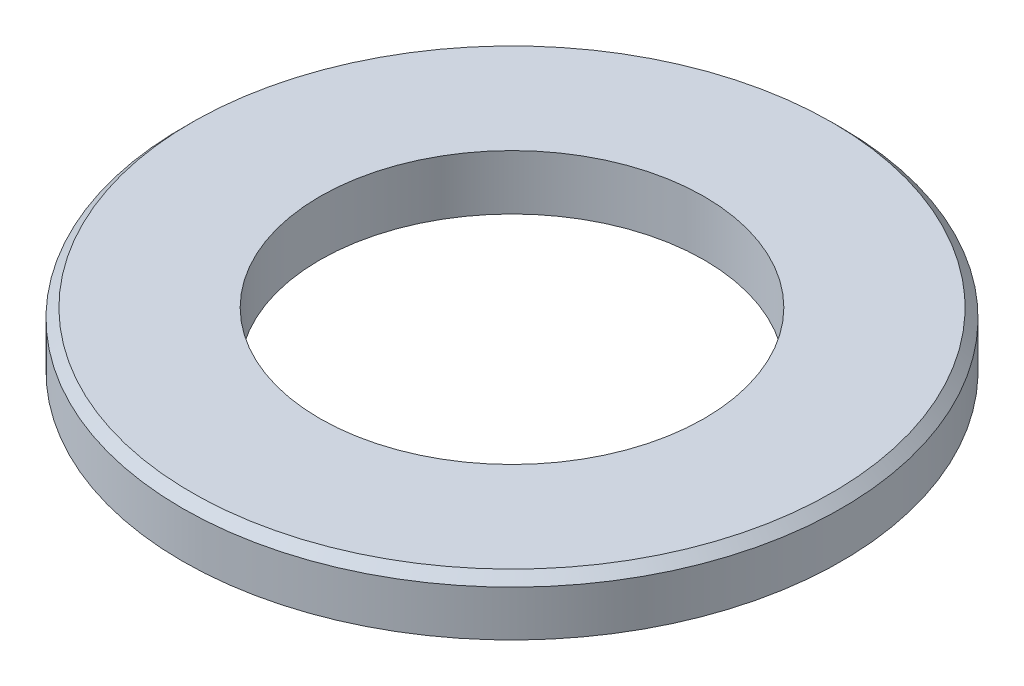
SolidWorks part; units mm, degrees
material "65Mn"
ref_plane "Plane1" through (0, 0, 0) normal (0, 0, 1) x (1, 0, 0)
ref_plane "Plane2" through (0, 0, 0) normal (0, 1, 0) x (1, 0, 0)
ref_plane "Plane3" through (0, 0, 0) normal (1, 0, 0) x (0, 0, -1)
sketch "Dimension sketch" plane through (0, 0, 0) normal (0, 0, 1) x (1, 0, 0)
  line L0 (0, 0) -> (9.1, 0)
  point P3 (4, 0)
  point P4 (56, 0)
  point P5 (31, 0)
  dimension "h" = 4
  dimension "d2" = 56
  dimension "d1" = 31
sketch "Sketch1" plane through (0, 0, 0) normal (0, 0, 1) x (1, 0, 0)
  line L0 (0, 0) -> (0, 52.7318) construction
  line L1 (-35, 14.6445) -> (-36, 13.6445)
  line L2 (-21, 8.6445) -> (-36, 8.6445)
  line L3 (-21, 8.6445) -> (-21, 14.6445)
  line L4 (-21, 14.6445) -> (-35, 14.6445)
  line L5 (-36, 8.6445) -> (-36, 13.6445)
  point P4 (-36, 14.6445)
  dimension "D1" = 42
  dimension "D2" = 36
  dimension "h" = 6
revolve "Base-Revolve" add sketch "Sketch1" angle 360 about L0
